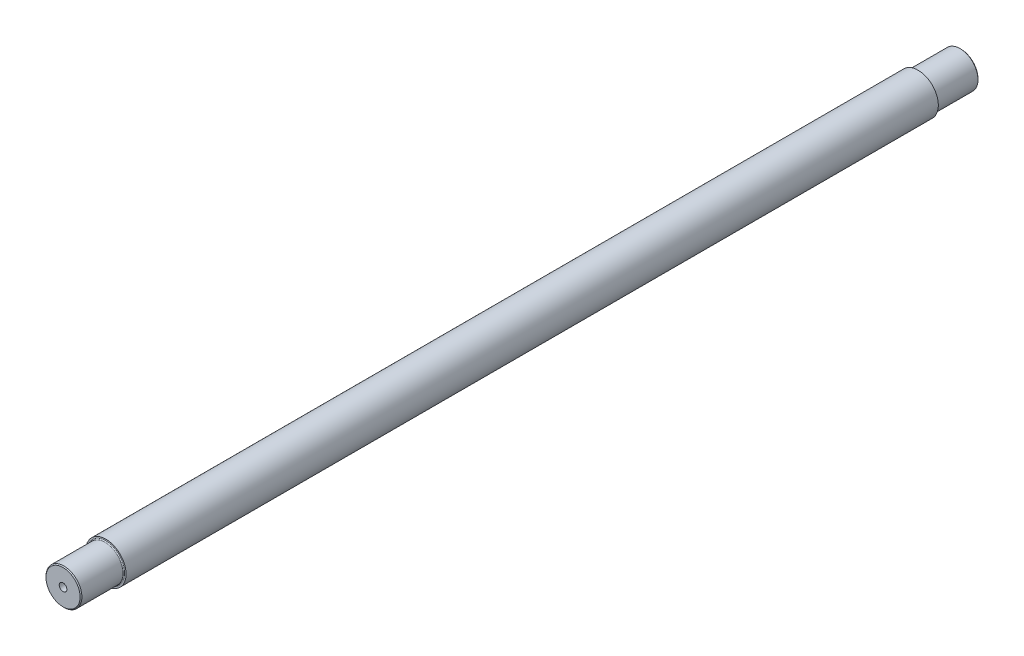
SolidWorks part; units mm, degrees
ref_plane "前视基准面" through (0, 0, 0) normal (0, 0, 1) x (1, 0, 0)
ref_plane "上视基准面" through (0, 0, 0) normal (0, 1, 0) x (1, 0, 0)
ref_plane "右视基准面" through (0, 0, 0) normal (1, 0, 0) x (0, 0, -1)
sketch "草图1" plane through (0, 0, 0) normal (0, 0, 1) x (1, 0, 0)
  circle A0 centre (0, 0) radius 22.5
  dimension "D1" = 45
extrude "凸台-拉伸1" add sketch "草图1" along normal blind 904.6
sketch "草图2" plane through (0, 0, 904.6) normal (0, 0, 1) x (1, 0, 0)
  circle A0 centre (0, 0) radius 20
  dimension "D1" = 40
extrude "凸台-拉伸2" add sketch "草图2" along normal blind 47.7 contours A0
sketch "草图3" plane through (0, 0, 0) normal (0, 0, -1) x (-1, 0, 0)
  circle A0 centre (0, 0) radius 20
  dimension "D1" = 40
extrude "凸台-拉伸3" add sketch "草图3" along normal blind 47.7
fillet "圆角1" radius 1 2 edges at (-20, 0, 0) (20, 0, 904.6)
chamfer "倒角1" distance 1 angle 45 2 edges at (20, 0, 952.3) (-20, 0, -47.7)
sketch "草图4" plane through (0, 0, 952.3) normal (0, 0, 1) x (1, 0, 0)
  circle A0 centre (0, 0) radius 5 construction
  dimension "D1" = 10
hole_wizard "M10 螺纹孔1" positions "草图5" profile "草图6" tap size "M10" standard "GB"
sketch "草图5" plane through (0, 0, 952.3) normal (0, 0, 1) x (1, 0, 0)
  point P0 (0, 0)
sketch "草图6" plane through (0, 0, 952.3) normal (1, 0, 0) x (0, -1, 0)
  line L0 (0, 0) -> (0, 27.0537)
  line L1 (0, 27.0537) -> (4.25, 24.5)
  line L2 (4.25, 24.5) -> (4.25, 0)
  line L5 (4.25, 0) -> (0, 0)
  line L10 (0, 27.0537) -> (-4.25, 24.5) construction
  line L11 (0, -6.35) -> (0, 107.95) construction
  dimension "螺纹孔钻头直径" = 8.5
  dimension "螺纹孔钻头深度" = 24.5
  dimension "导头角度" = 118
cosmetic thread "孔螺蚊线1" parameters "D1"=20, "D2"=10
sketch "草图7" plane through (0, 0, -47.7) normal (0, 0, -1) x (-1, 0, 0)
  circle A0 centre (0, 0) radius 5 construction
  dimension "D1" = 10
hole_wizard "M10 螺纹孔2" positions "草图8" profile "草图9" tap size "M10" standard "GB"
sketch "草图8" plane through (0, 0, -47.7) normal (0, 0, -1) x (-1, 0, 0)
  point P0 (0, 0)
sketch "草图9" plane through (0, 0, -47.7) normal (1, 0, 0) x (0, 1, 0)
  line L0 (0, 0) -> (0, 27.0537)
  line L1 (0, 27.0537) -> (4.25, 24.5)
  line L2 (4.25, 24.5) -> (4.25, 0)
  line L5 (4.25, 0) -> (0, 0)
  line L10 (0, 27.0537) -> (-4.25, 24.5) construction
  line L11 (0, -6.35) -> (0, 107.95) construction
  dimension "螺纹孔钻头直径" = 8.5
  dimension "螺纹孔钻头深度" = 24.5
  dimension "导头角度" = 118
cosmetic thread "孔螺蚊线2" parameters "D1"=20, "D2"=10
